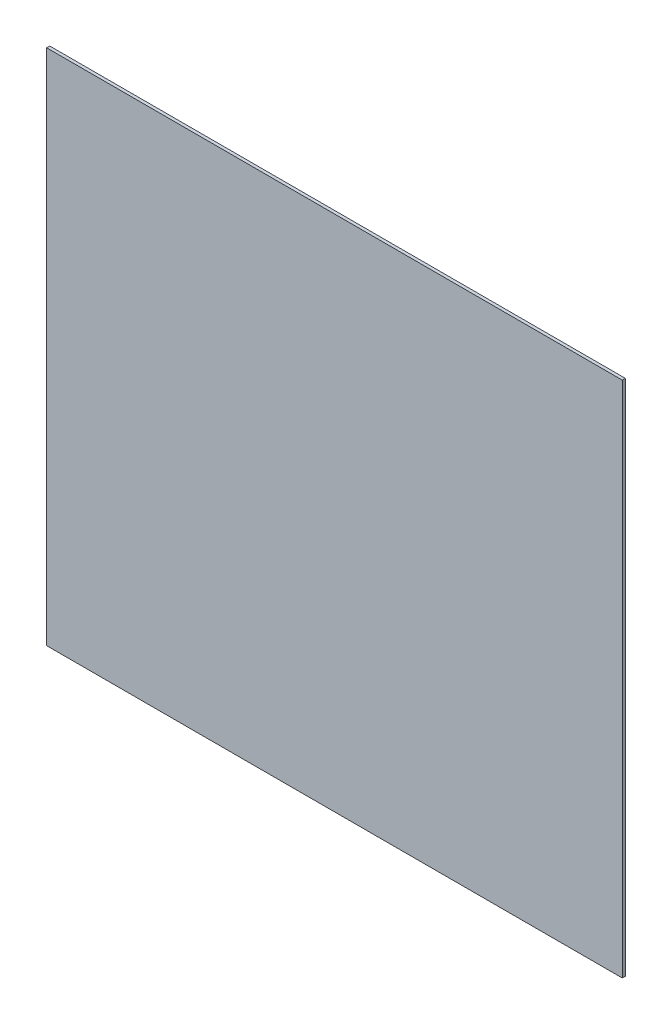
from build123d import *

# Parameters (mm, degrees)
SKETCH_1_W      = 936
SKETCH_1_H      = 842
EXTRUDE_1_DEPTH = 5


with BuildPart() as part:
    # 草图1 → 凸台-拉伸1 (new body)
    with BuildSketch(Plane.XY):
        Rectangle(SKETCH_1_W, SKETCH_1_H)
    extrude(amount=EXTRUDE_1_DEPTH)


solid = part.part
